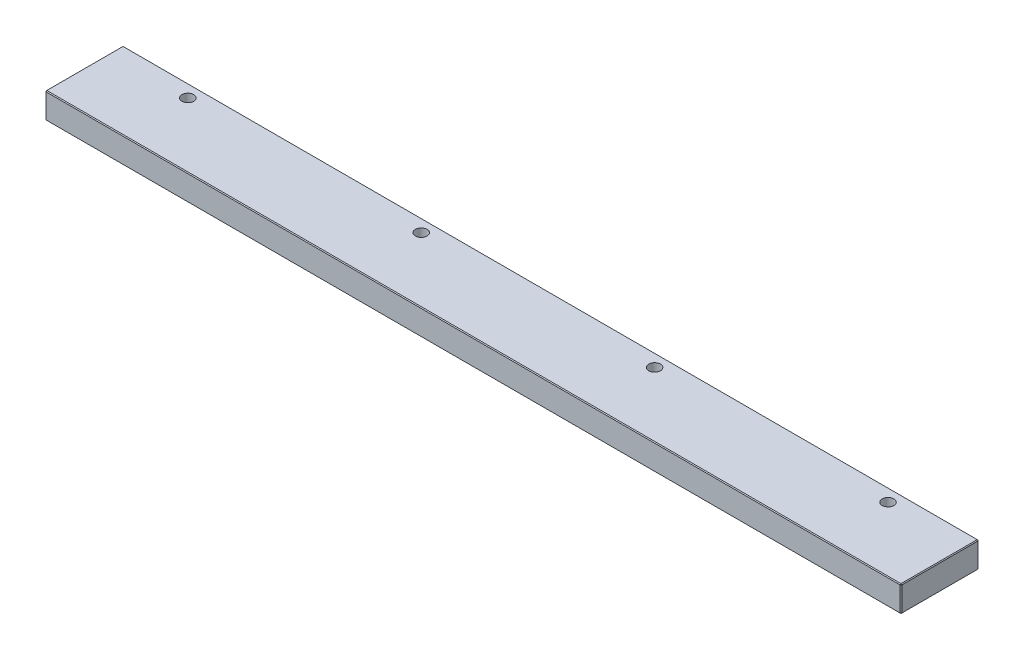
SolidWorks part; units mm, degrees
ref_plane "Front" through (0, 0, 0) normal (0, 0, 1) x (1, 0, 0)
ref_plane "Top" through (0, 0, 0) normal (0, 1, 0) x (1, 0, 0)
ref_plane "Right" through (0, 0, 0) normal (1, 0, 0) x (0, 0, -1)
sketch "草图1" plane through (0, 0, 0) normal (0, 1, 0) x (1, 0, 0)
  line L1 (-165, 15) -> (165, 15)
  line L2 (-165, 15) -> (-165, -15)
  line L3 (-165, -15) -> (165, -15)
  line L4 (165, 15) -> (165, -15)
  line L5 (-165, 15) -> (165, -15) construction
  line L6 (-165, -15) -> (165, 15) construction
  point P0 (0, 0)
  dimension "D1" = 30
  dimension "D2" = 330
extrude "凸台-拉伸1" add sketch "草图1" along normal blind 10
hole_wizard "M4 六角凹头螺钉的柱形沉头孔1" positions "草图3" profile "草图2" counterbore size "M4" standard "Iso" end condition through all
sketch "草图3" plane through (0, 0, 0) normal (0, -1, 0) x (-1, 0, 0)
  line L0 (0, 0) -> (0, 15) construction
  line L1 (-165, 15) -> (165, 15) construction
  point P0 (-135, 10)
  point P2 (-45, 10)
  point P4 (45, 10)
  point P6 (135, 10)
  dimension "D1" = 90
  dimension "D2" = 90
  dimension "D3" = 5
sketch "草图2" plane through (135, 0, -10) normal (1, 0, 0) x (0, 0, -1)
  line L0 (0, 0) -> (0, 10)
  line L1 (0, 10) -> (2.25, 10)
  line L3 (2.25, 10) -> (2.25, 4.4)
  line L4 (2.25, 4.4) -> (4, 4.4)
  line L5 (4, 4.4) -> (4, 0)
  line L7 (4, 0) -> (0, 0)
  line L11 (0, -6.35) -> (0, 107.95) construction
  dimension "通孔孔直径" = 4.5
  dimension "通孔孔深度" = 10
  dimension "柱形沉头孔直径" = 8
  dimension "柱形沉头孔深度" = 4.4
chamfer "倒角1" distance 0.3 angle 45 12 edges at (165, 10, 0) (165, 0, 0) (0, 10, 15) (165, 5, 15) (0, 0, 15) (-165, 10, 0) (-165, 5, 15) (-165, 0, 0) (165, 5, -15) (0, 10, -15) (-165, 5, -15) (0, 0, -15)
